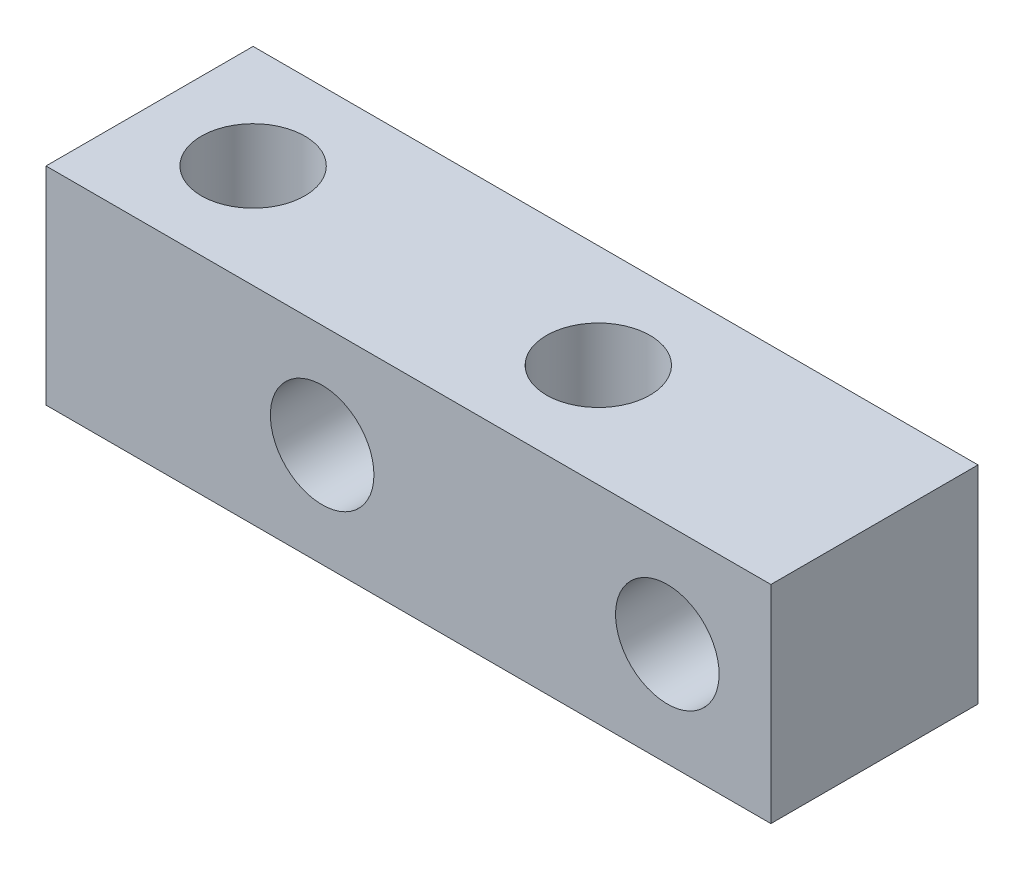
SolidWorks part; units mm, degrees
material "6061 合金"
ref_plane "前视基准面" through (0, 0, 0) normal (0, 0, 1) x (1, 0, 0)
ref_plane "上视基准面" through (0, 0, 0) normal (0, 1, 0) x (1, 0, 0)
ref_plane "右视基准面" through (0, 0, 0) normal (1, 0, 0) x (0, 0, -1)
other "Configuration Table"
sketch "草图1" plane through (0, 0, 0) normal (0, 1, 0) x (1, 0, 0)
  line L1 (0, 0) -> (21, 0)
  line L2 (0, 0) -> (0, 6)
  line L3 (0, 6) -> (21, 6)
  line L4 (21, 0) -> (21, 6)
  circle A0 centre (3, 3) radius 1.5
  circle A1 centre (13, 3) radius 1.5
  dimension "D3" = 3
  dimension "D4" = 3
  dimension "D5" = 3
  dimension "D6" = 3
  dimension "D7" = 10
  dimension "D8" = 3
  dimension "D1" = 21
  dimension "D2" = 6
extrude "凸台-拉伸1" add sketch "草图1" along normal blind 6
sketch "草图2" plane through (0, 0, 0) normal (0, 0, 1) x (1, 0, 0)
  line L0 (21, 3) -> (0, 3) construction
  line L1 (21, 6) -> (21, 0) construction
  line L2 (0, 6) -> (0, 0) construction
  circle A0 centre (18, 3) radius 1.5
  circle A1 centre (8, 3) radius 1.5
  dimension "D1" = 3
  dimension "D2" = 3
  dimension "D3" = 3
  dimension "D4" = 10
extrude "切除-拉伸1" cut sketch "草图2" against normal through all
